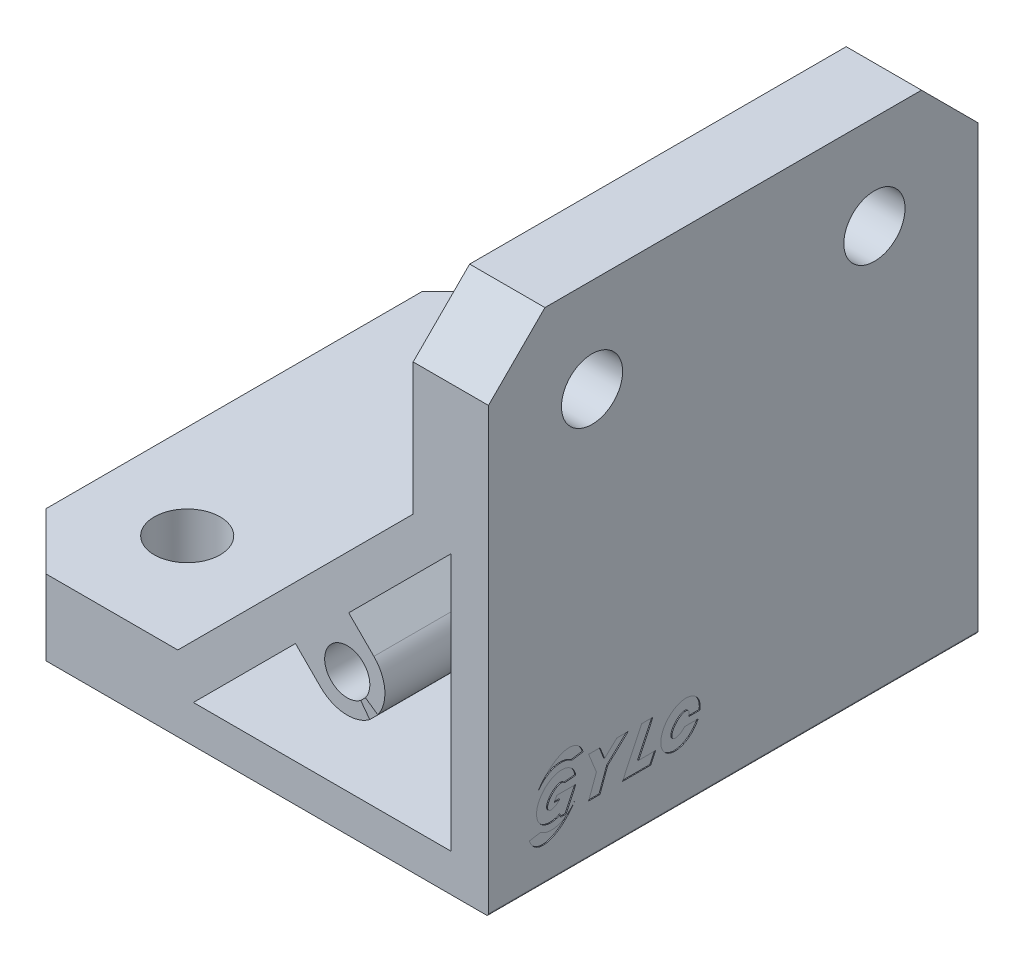
from build123d import *

# Parameters (mm, degrees)
EXTRUDE_1_DEPTH     = 52
SKETCH_1_R          = 3.5
CUT_EXTRUDE_1_DEPTH = 10
SKETCH_3_R          = 3.25
CUT_EXTRUDE_2_DEPTH = 10
CUT_EXTRUDE_3_DEPTH = 0.1
CHAMFER_2_SIZE      = 6


with BuildPart() as part:
    # Model → 凸台-拉伸1 (new body)
    with BuildSketch(Plane.XY):
        with BuildLine():
            Line((376.14070145, 195.588546008), (384.14070145, 195.588546008))
            Line((384.14070145, 195.588546008), (384.14070145, 142.825500368))
            ThreePointArc((384.14070145, 142.825500368), (384.071299125, 142.657948334), (383.90374709, 142.588546008))
            Line((383.90374709, 142.588546008), (331.14070145, 142.588546008))
            Line((331.14070145, 142.588546008), (331.14070145, 150.588546008))
            Line((331.14070145, 150.588546008), (351.14070145, 150.588546008))
            Line((351.14070145, 150.588546008), (376.14070145, 175.588546008))
            Line((376.14070145, 175.588546008), (376.14070145, 195.588546008))
        make_face()
        with BuildLine():
            Line((352.797555699, 146.588546008), (380.14070145, 146.588546008))
            Line((380.14070145, 146.588546008), (380.14070145, 173.931691759))
            Line((380.14070145, 173.931691759), (369.297555699, 163.088546008))
            Line((369.297555699, 163.088546008), (371.969128574, 160.416973133))
            ThreePointArc((371.969128574, 160.416973133), (373.12775021, 157.910170293), (372.385928963, 155.25006394))
            Line((372.385928963, 155.25006394), (371.072213777, 156.164024991))
            ThreePointArc((371.072213777, 156.164024991), (367.439726654, 159.281674694), (370.574137304, 155.663640387))
            Line((370.574137304, 155.663640387), (371.529761206, 154.380369972))
            ThreePointArc((371.529761206, 154.380369972), (368.850334045, 153.599099083), (366.312274325, 154.760118884))
            Line((366.312274325, 154.760118884), (363.64070145, 157.431691759))
            Line((363.64070145, 157.431691759), (352.797555699, 146.588546008))
        make_face(mode=Mode.SUBTRACT)
    extrude(amount=EXTRUDE_1_DEPTH)

    # 草图1 → 切除-拉伸1 (cut)
    with BuildSketch(Plane(origin=(0, 142.588546008, 0), x_dir=(-1, 0, 0), z_dir=(0, -1, 0))):
        with Locations(Location((-341.14070145, -11, 0), (0, 0, 90))):
            Circle(SKETCH_1_R)
        with Locations(Location((-341.14070145, -41, 0), (0, 0, 90))):
            Circle(SKETCH_1_R)
    extrude(amount=-CUT_EXTRUDE_1_DEPTH, mode=Mode.SUBTRACT)

    # 草图3 → 切除-拉伸2 (cut)
    with BuildSketch(Plane(origin=(384.14070145, 0, 0), x_dir=(0, 0, -1), z_dir=(1, 0, 0))):
        with Locations((-41, 185.588546008)):
            Circle(SKETCH_3_R)
        with Locations((-11, 185.588546008)):
            Circle(SKETCH_3_R)
    extrude(amount=-CUT_EXTRUDE_2_DEPTH, mode=Mode.SUBTRACT)

    # 草图4 → 切除-拉伸3 (cut)
    with BuildSketch(Plane(origin=(384.14070145, 0, 0), x_dir=(0, 0, -1), z_dir=(1, 0, 0))):
        with BuildLine():
            Line((-31.156910998, 149.620936237), (-29.734918025, 149.620936237))
            add(Edge.make_bspline(
                [(-29.527213106, 150.324263564), (-29.069640514, 153.582209756), (-32.160166716, 151.852897671), (-35.250692919, 150.123585587), (-33.22217607, 148.256737296), (-31.193659222, 146.389889004), (-29.734918025, 149.620936237)],
                knots=[2.310776883, 2.310776883, 2.310776883, 4.295504112, 4.295504112, 6.280231341, 6.280231341, 8.26495857, 8.26495857, 8.26495857], degree=2, weights=[1, 0.546712287, 1, 0.546712287, 1, 0.546712287, 1]))
            Line((-29.527213106, 150.324263564), (-30.727213106, 150.324263564))
            add(Edge.make_bspline(
                [(-30.727213106, 150.324263564), (-30.331693937, 151.551759326), (-31.551251149, 150.835698352), (-32.770808361, 150.119637377), (-32.499443953, 149.28370119), (-32.228079545, 148.447765002), (-31.156910998, 149.620936237)],
                knots=[2.310776883, 2.310776883, 2.310776883, 4.1585118, 4.1585118, 6.006246717, 6.006246717, 7.853981634, 7.853981634, 7.853981634], degree=2, weights=[1, 0.602738677, 1, 0.602738677, 1, 0.602738677, 1]))
        make_face()
        with BuildLine():
            Line((-43.925569034, 150.826737427), (-42.730135397, 150.931324318))
            add(Edge.make_bspline(
                [(-42.730135397, 150.931324318), (-43.532943041, 155.84269164), (-46.525470552, 150.700825597), (-49.517998063, 145.558959554), (-44.356910998, 148.136141251)],
                knots=[2.606547406, 2.606547406, 2.606547406, 4.993026489, 4.993026489, 7.379505572, 7.379505572, 7.379505572], degree=2, weights=[1, 0.368650437, 1, 0.368650437, 1]))
            Line((-44.356910998, 148.136141251), (-44.356910998, 147.877409345))
            Line((-44.356910998, 147.877409345), (-43.756910998, 147.877409345))
            Line((-43.756910998, 147.877409345), (-42.713374, 150.089660335))
            Line((-42.713374, 150.089660335), (-44.741418493, 150.089660335))
            Line((-44.741418493, 150.089660335), (-45.017517564, 149.556960323))
            Line((-45.017517564, 149.556960323), (-44.417517564, 149.556960323))
            add(Edge.make_bspline(
                [(-43.925569034, 150.826737427), (-44.690411989, 152.268585428), (-45.646229095, 149.801508889), (-46.602046201, 147.334432349), (-44.417517564, 149.556960323)],
                knots=[2.964843337, 2.964843337, 2.964843337, 5.372666732, 5.372666732, 7.780490127, 7.780490127, 7.780490127], degree=2, weights=[1, 0.358709137, 1, 0.358709137, 1]))
        make_face()
        Polygon((-41.356910998, 147.877409345), (-40.156910998, 147.877409345), (-39.336062654, 150.132671635), (-37.156910998, 152.173591391), (-38.356910998, 152.173591391), (-39.664401992, 150.949039538), (-40.156910998, 152.173591391), (-41.356910998, 152.173591391), (-40.536062654, 150.132671635), align=None)
        Polygon((-35.73036657, 152.173591391), (-37.756910998, 147.877409345), (-34.756910998, 147.877409345), (-34.244959606, 148.96272302), (-36.044959606, 148.96272302), (-34.53036657, 152.173591391), align=None)
        with BuildLine():
            Line((-43.130690832, 152.515854721), (-41.945152764, 152.701595103))
            add(Edge.make_bspline(
                [(-41.945152764, 152.701595103), (-43.36499983, 157.051657906), (-46.85513293, 151.265027956)],
                knots=[2.682976295, 2.682976295, 2.682976295, 4.71238898, 4.71238898, 4.71238898], degree=2, weights=[1, 0.527869365, 1]))
            add(Edge.make_bspline(
                [(-43.130690832, 152.515854721), (-45.210313594, 153.992133359), (-46.85513293, 151.265027956)],
                knots=[6.223464168, 6.223464168, 6.223464168, 7.853981634, 7.853981634, 7.853981634], degree=2, weights=[1, 0.685680084, 1]))
        make_face()
        with BuildLine():
            Line((-47.654847236, 147.349405634), (-46.469309168, 147.535146015))
            add(Edge.make_bspline(
                [(-46.469309168, 147.535146015), (-44.389686406, 146.058867378), (-42.74486707, 148.78597278)],
                knots=[3.081871514, 3.081871514, 3.081871514, 4.71238898, 4.71238898, 4.71238898], degree=2, weights=[1, 0.685680084, 1]))
            add(Edge.make_bspline(
                [(-47.654847236, 147.349405634), (-46.23500017, 142.999342831), (-42.74486707, 148.78597278)],
                knots=[2.682976295, 2.682976295, 2.682976295, 4.71238898, 4.71238898, 4.71238898], degree=2, weights=[1, 0.527869365, 1]))
        make_face()
    extrude(amount=-CUT_EXTRUDE_3_DEPTH, mode=Mode.SUBTRACT)

    # 倒角2
    chamfer_2_edges = [part.edges().sort_by_distance(p)[0] for p in [
        (331.14070145, 146.588546008, 52),
        (380.14070145, 195.588546008, 52),
        (380.14070145, 195.588546008, 0),
        (331.14070145, 146.588546008, 0),
    ]]
    chamfer(chamfer_2_edges, length=CHAMFER_2_SIZE)


solid = part.part
